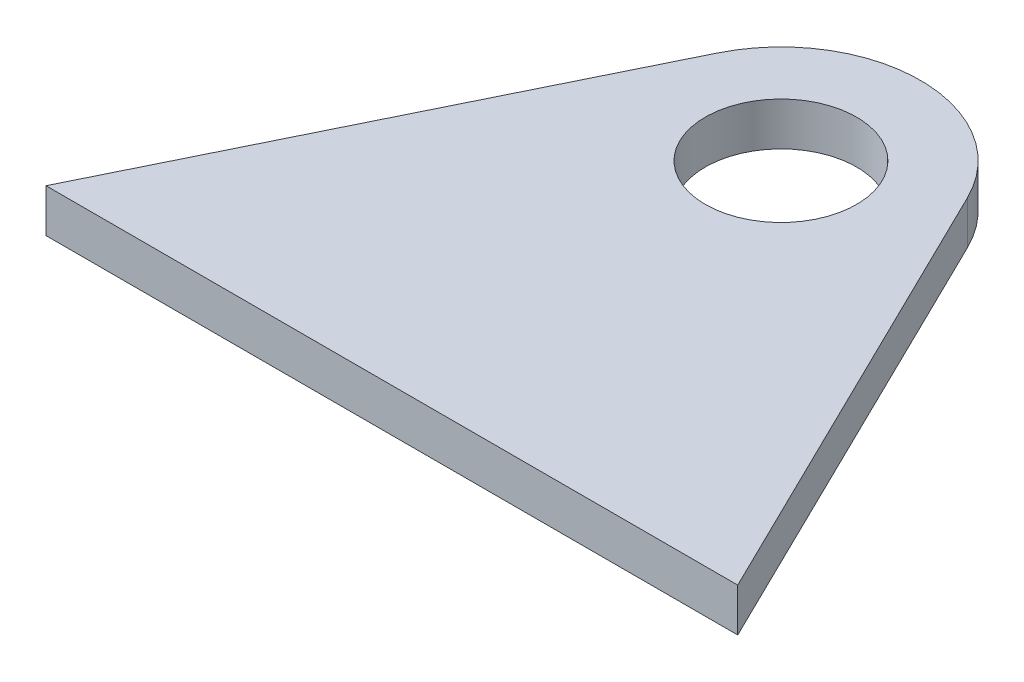
SolidWorks part; units mm, degrees
ref_plane "前视基准面" through (0, 0, 0) normal (0, 0, 1) x (1, 0, 0)
ref_plane "上视基准面" through (0, 0, 0) normal (0, 1, 0) x (1, 0, 0)
ref_plane "右视基准面" through (0, 0, 0) normal (1, 0, 0) x (0, 0, -1)
sketch "草图1" plane through (0, 0, 0) normal (0, 1, 0) x (1, 0, 0)
  line L0 (0, 0) -> (160, 0)
  line L3 (0, 0) -> (51.0383, 104.1875)
  line L4 (160, 0) -> (108.9617, 104.1875)
  circle A0 centre (80, 90) radius 17.25
  arc A1 (108.9617, 104.1875) -> (51.0383, 104.1875) centre (80, 90) ccw
extrude "凸台-拉伸1" add sketch "草图1" along normal blind 10
sketch "草图2" plane through (0, 10, 0) normal (0, 1, 0) x (1, 0, 0)
  circle A1 centre (80, 90) radius 17.5
extrude "切除-拉伸1" cut sketch "草图2" against normal blind 10
